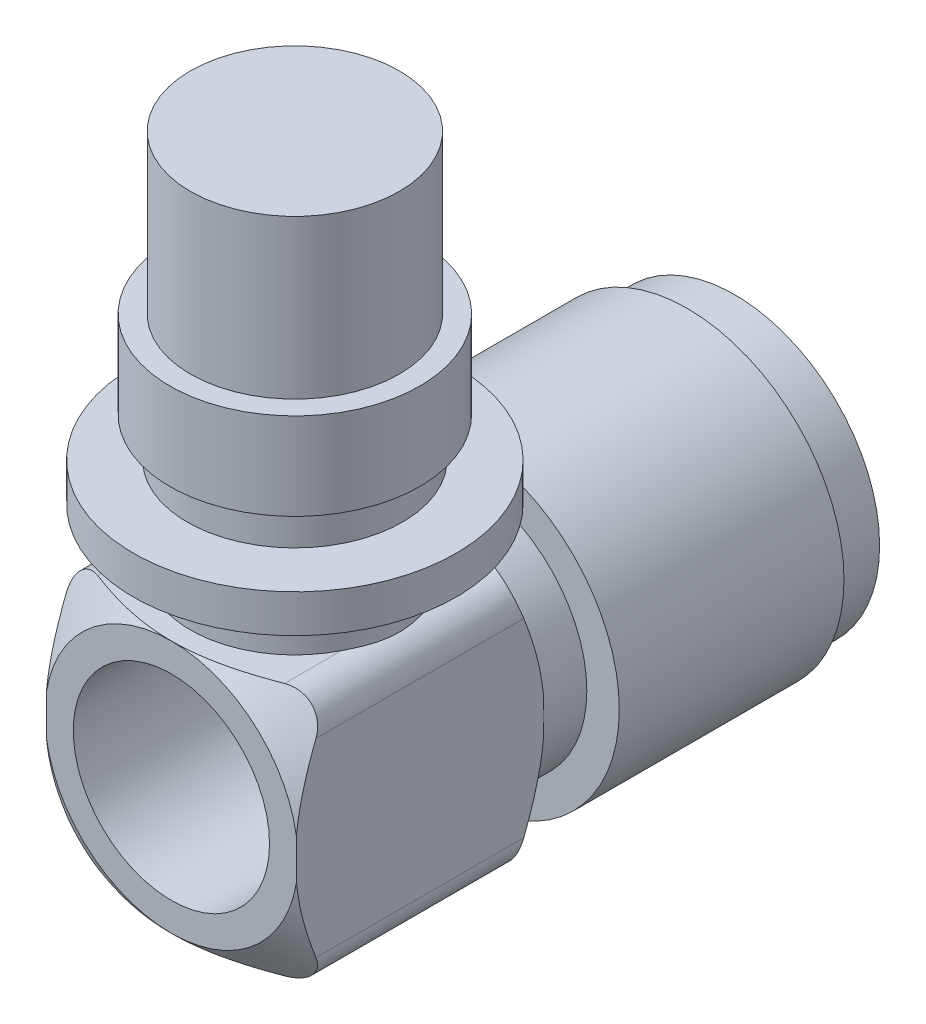
from build123d import *

# Parameters (mm, degrees)
SKETCH1_W           = 7.9
SKETCH1_H           = 7.8
BOSS_EXTRUDE1_DEPTH = 8
FILLET1_R           = 1
BOSS_EXTRUDE2_REACH = 22.756
SKETCH4_R           = 3.3
SKETCH6_R           = 3.925
BOSS_EXTRUDE3_DEPTH = 6.75
SKETCH9_R           = 3.1
CUT_EXTRUDE1_DEPTH  = 5


with BuildPart() as part:
    # Sketch1 → Boss-Extrude1 (new body)
    with BuildSketch(Plane(origin=(0, 0, 0), x_dir=(1, 0, 0), z_dir=(0, 1, 0))):
        Rectangle(SKETCH1_W, SKETCH1_H)
    extrude(amount=BOSS_EXTRUDE1_DEPTH)

    # Fillet1
    fillet1_edges = [part.edges().sort_by_distance(p)[0] for p in [
        (-3.95, 8, 0),
        (3.95, 8, 0),
        (-3.95, 0, 0),
        (3.95, 0, 0),
    ]]
    fillet(fillet1_edges, radius=FILLET1_R)

    # Sketch3 → Cut-Revolve4 (revolve, cut)
    with BuildSketch(Plane(origin=(-2, 2, 0), x_dir=(0, 0, -1), z_dir=(0.7071067811865462, -0.7071067811865488, 0))):
        Polygon((3, 8.228427125), (4, 8.228427125), (3.9, 6.828427125), align=None)
    cut_revolve4 = revolve(axis=Axis((0, 4, 3.9), (0, 0, -1)), mode=Mode.SUBTRACT)

    # Mirror2: Cut-Revolve4 across plane
    add(cut_revolve4.mirror(Plane.XY), mode=Mode.SUBTRACT)

    # Sketch4 → Boss-Extrude2 (add, up to next)
    with BuildSketch(Plane(origin=(0, 20, 0), x_dir=(1, 0, 0), z_dir=(0, 1, 0)), mode=Mode.PRIVATE) as boss_extrude2_sk1:
        with Locations(Location((0, 0, 0), (0, 0, 270))):
            Circle(SKETCH4_R)
    boss_extrude2_tool1 = extrude(boss_extrude2_sk1.sketch, amount=-BOSS_EXTRUDE2_REACH, mode=Mode.PRIVATE) - part.part
    add(boss_extrude2_tool1.solids().sort_by_distance((0, 20, 0))[0])

    # Sketch5 → Revolve1 (revolve)
    with BuildSketch(Plane(origin=(0, 0, 0), x_dir=(0, 0, -1), z_dir=(1, 0, 0)), mode=Mode.PRIVATE) as revolve1_sk:
        Polygon((-5.1, 11), (-5.1, 9.8), (-3.3, 9.8), (-3.3, 15), (-3.95, 15), (-3.95, 12.25), (-3.4, 12.25), (-3.4, 11), align=None)
    revolve(revolve1_sk.sketch.rotate(Axis((0, -3.247015834, 0), (0, 1, 0)), 180), axis=Axis((0, -3.247015834, 0), (0, 1, 0)))

    # Sketch6 → Boss-Extrude3 (add)
    with BuildSketch(Plane(origin=(0, 0, -3.9), x_dir=(-1, 0, 0), z_dir=(0, 0, -1))):
        with Locations(Location((0, 4, 0), (0, 0, 180))):
            Circle(SKETCH6_R)
    extrude(amount=BOSS_EXTRUDE3_DEPTH)

    # Sketch8 → Revolve2 (revolve)
    with BuildSketch(Plane(origin=(0, 0, 0), x_dir=(0, 0, -1), z_dir=(1, 0, 0)), mode=Mode.PRIVATE) as revolve2_sk:
        Polygon((5.3, 4), (5.3, 8.95), (12.4, 8.95), (12.4, 8.575), (13.9, 8.575), (13.9, 7.6875), (13.4, 7.6875), (12.887601636, 6.8), (10.65, 6.8), (10.65, 4.470320629), (12.385380774, 4.470320629), (13.2, 4), align=None)
    revolve(revolve2_sk.sketch.rotate(Axis((0, 4, 5.444048586), (0, 0, -1)), 90), axis=Axis((0, 4, 5.444048586), (0, 0, -1)))

    # Sketch9 → Cut-Extrude1 (cut)
    with BuildSketch(Plane.XY.offset(3.9)):
        with Locations((0, 4)):
            Circle(SKETCH9_R)
    extrude(amount=-CUT_EXTRUDE1_DEPTH, mode=Mode.SUBTRACT)


solid = part.part
